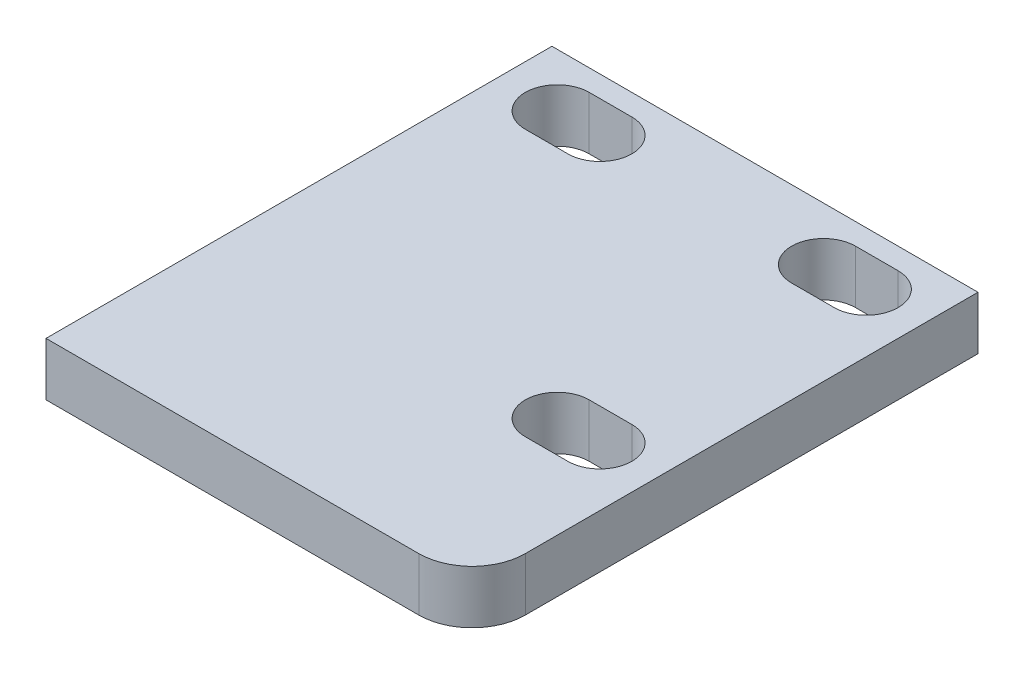
SolidWorks part; units mm, degrees
material "Q235B"
ref_plane "Front Plane" through (0, 0, 0) normal (0, 0, 1) x (1, 0, 0)
ref_plane "Top Plane" through (0, 0, 0) normal (0, 1, 0) x (1, 0, 0)
ref_plane "Right Plane" through (0, 0, 0) normal (1, 0, 0) x (0, 0, -1)
other "Configuration Table"
sketch "Sketch1" plane through (0, 0, 0) normal (0, 1, 0) x (1, 0, 0)
  line L0 (-29, 37.5) -> (-21, 37.5) construction
  line L1 (-40, -47.5) -> (30, -47.5)
  line L2 (-40, -47.5) -> (-40, 47.5)
  line L3 (-40, 47.5) -> (40, 47.5)
  line L4 (40, -37.5) -> (40, 47.5)
  line L5 (-40, -47.5) -> (40, 47.5) construction
  line L6 (-40, 47.5) -> (40, -47.5) construction
  line L7 (-29, 43.5) -> (-21, 43.5)
  line L8 (-29, 31.5) -> (-21, 31.5)
  line L9 (21, 31.5) -> (29, 31.5)
  line L12 (0, 0) -> (0, 13.3993) construction
  line L13 (21, 43.5) -> (29, 43.5)
  line L14 (21, 37.5) -> (29, 37.5) construction
  line L15 (21, -18.5) -> (29, -18.5)
  line L16 (21, -6.5) -> (29, -6.5)
  line L17 (21, -12.5) -> (29, -12.5) construction
  line L21 (-29, -6.5) -> (-21, -6.5) [skipped]
  line L22 (-29, -18.5) -> (-21, -18.5) [skipped]
  arc A0 (-29, 43.5) -> (-29, 31.5) centre (-29, 37.5) ccw
  arc A1 (-21, 31.5) -> (-21, 43.5) centre (-21, 37.5) ccw
  arc A4 (21, 43.5) -> (21, 31.5) centre (21, 37.5) ccw
  arc A5 (29, 31.5) -> (29, 43.5) centre (29, 37.5) ccw
  arc A6 (21, -6.5) -> (21, -18.5) centre (21, -12.5) ccw
  arc A7 (29, -18.5) -> (29, -6.5) centre (29, -12.5) ccw
  arc A10 (-29, -6.5) -> (-29, -18.5) centre (-29, -12.5) ccw [skipped]
  arc A11 (-21, -18.5) -> (-21, -6.5) centre (-21, -12.5) ccw [skipped]
  arc A12 (30, -47.5) -> (40, -37.5) centre (30, -37.5) ccw
  point P0 (0, 0)
  point P8 (-25, 37.5)
  point P17 (25, 37.5)
  point P22 (-35, 37.5)
  point P23 (-15, 37.5)
  point P24 (-25, 43.5)
  point P29 (25, -12.5)
  dimension "D5" = 6
  dimension "D9" = 10
  dimension "D1" = 80
  dimension "D2" = 95
  dimension "D3" = 10
  dimension "D4" = 20
  dimension "D6" = 15
  dimension "D7" = 2
  dimension "D8" = 2
extrude "Boss-Extrude1" add sketch "Sketch1" along normal blind 10
